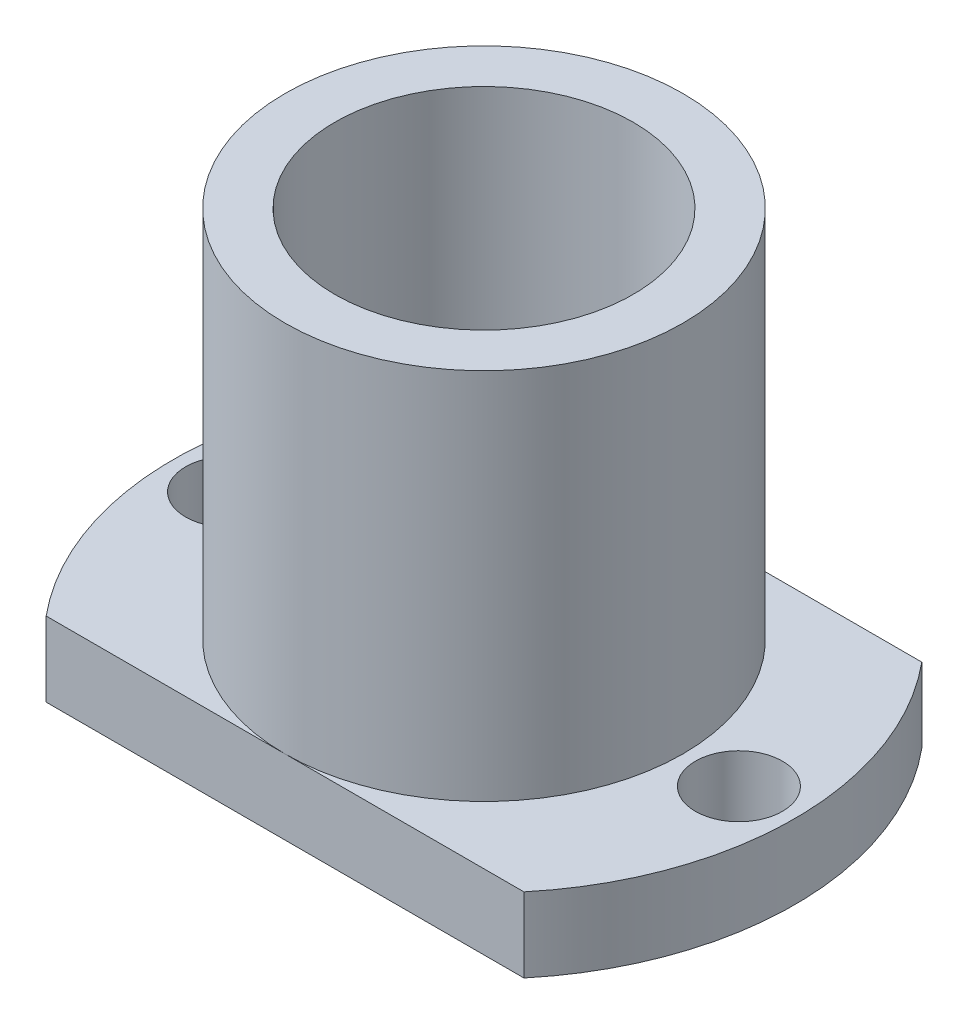
SolidWorks part; units mm, degrees
ref_plane "Front Plane" through (0, 0, 0) normal (0, 0, 1) x (1, 0, 0)
ref_plane "Top Plane" through (0, 0, 0) normal (0, 1, 0) x (1, 0, 0)
ref_plane "Right Plane" through (0, 0, 0) normal (1, 0, 0) x (0, 0, -1)
sketch "Sketch1" plane through (0, 0, 0) normal (0, 0, 1) x (1, 0, 0)
  line L0 (0, 0) -> (0, 40.9444) construction
  line L1 (12, 36) -> (12, 0)
  line L2 (12, 0) -> (25, 0)
  line L3 (25, 0) -> (25, 6)
  line L4 (25, 6) -> (16, 6)
  line L5 (16, 6) -> (16, 36)
  line L6 (16, 36) -> (12, 36)
  dimension "D1" = 16
  dimension "D2" = 4
  dimension "D3" = 6
  dimension "D4" = 25
  dimension "D5" = 36
revolve "Revolve1" add sketch "Sketch1" angle 360 about L0
sketch "Sketch2" plane through (0, 6, 0) normal (0, 1, 0) x (1, 0, 0)
  line L0 (-25, 0) -> (25, 0) construction
  line L1 (0, 25) -> (0, -25) construction
  circle A0 centre (0, 0) radius 25 construction
  circle A1 centre (0, 0) radius 20.5 construction
  circle A2 centre (-20.5, 0) radius 3.5
  circle A3 centre (0, 20.5) radius 3.5
  circle A4 centre (20.5, 0) radius 3.5
  circle A5 centre (0, -20.5) radius 3.5
  point P21 (0, 0)
  dimension "D1" = 41
  dimension "D2" = 7
  dimension "D3" = 4
extrude "Cut-Extrude1" cut sketch "Sketch2" against normal through all
sketch "Sketch3" plane through (0, 6, 0) normal (0, 1, 0) x (1, 0, 0)
  line L0 (-19.2094, 16) -> (19.2094, 16)
  line L1 (-19.2094, -16) -> (19.2094, -16)
  circle A0 centre (0, 0) radius 25 construction
  circle A1 centre (0, 0) radius 16 construction
  circle A2 centre (0, 0) radius 16 construction
  arc A3 (-19.2094, -16) -> (19.2094, -16) centre (0, 0) ccw
  arc A4 (19.2094, 16) -> (-19.2094, 16) centre (0, 0) ccw
extrude "Cut-Extrude2" cut sketch "Sketch3" against normal through all
